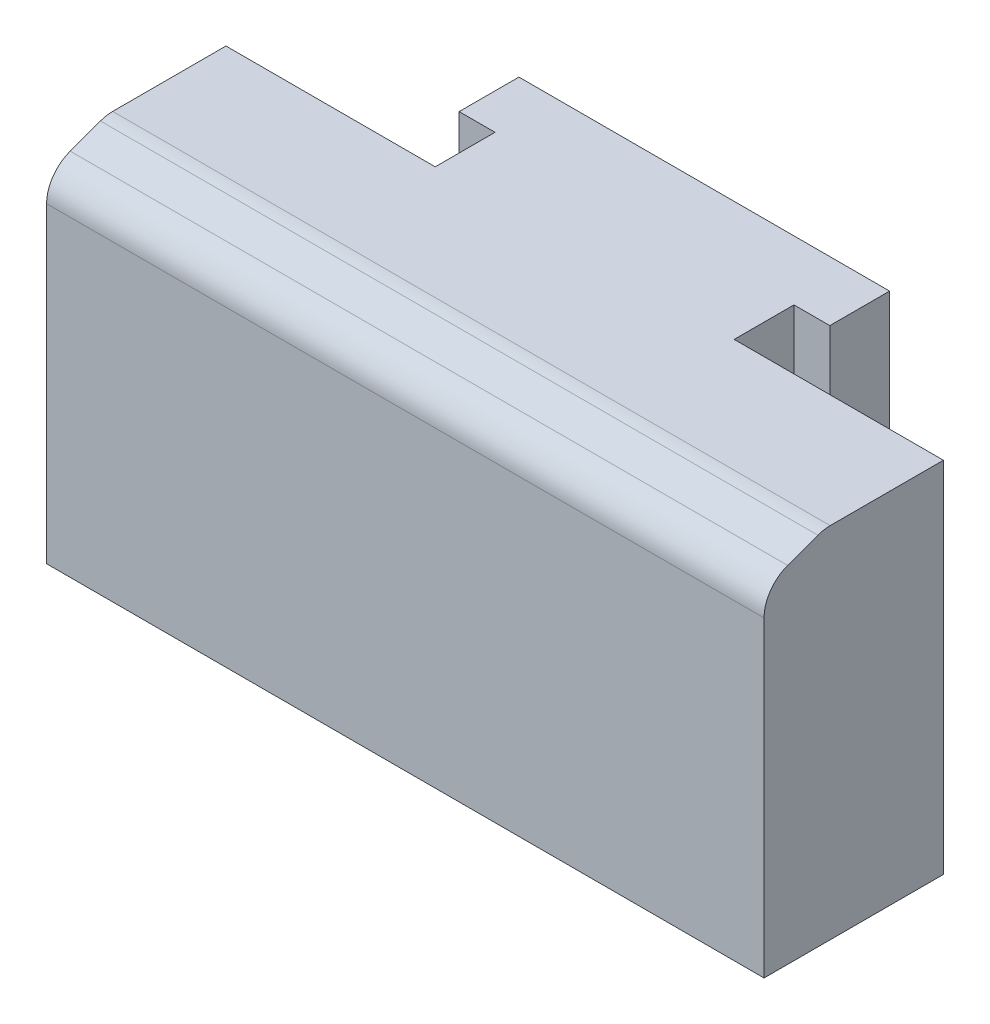
SolidWorks part; units mm, degrees
ref_plane "Front Plane" through (0, 0, 0) normal (0, 0, 1) x (1, 0, 0)
ref_plane "Top Plane" through (0, 0, 0) normal (0, 1, 0) x (1, 0, 0)
ref_plane "Right Plane" through (0, 0, 0) normal (1, 0, 0) x (0, 0, -1)
sketch "Sketch1" plane through (0, 0, 0) normal (0, 0, 1) x (1, 0, 0)
  line L1 (-32.0165, 30.1974) -> (-1.0165, 30.1974)
  line L2 (-32.0165, 30.1974) -> (-32.0165, 0.1974)
  line L3 (-32.0165, 0.1974) -> (-1.0165, 0.1974)
  line L4 (-1.0165, 30.1974) -> (-1.0165, 0.1974)
  dimension "D1" = 30
  dimension "D2" = 31
extrude "Boss-Extrude1" add sketch "Sketch1" along normal blind 25
sketch "Sketch2" plane through (0, 0.1974, 0) normal (0, -1, 0) x (1, 0, 0)
  line L0 (-32.0165, 25) -> (-1.0165, 25) construction
  line L5 (-16.5165, 0) -> (-16.5165, 13.8579) construction
  line L6 (-32.0165, 0) -> (-1.0165, 0) construction
  line L8 (-29.0165, 5) -> (-32.0165, 5)
  line L9 (-29.0165, 5) -> (-29.0165, 25)
  line L10 (-29.0165, 25) -> (-32.0165, 25)
  line L11 (-32.0165, 5) -> (-32.0165, 25)
  line L12 (-4.0165, 5) -> (-1.0165, 5)
  line L13 (-4.0165, 5) -> (-4.0165, 25)
  line L14 (-4.0165, 25) -> (-1.0165, 25)
  line L15 (-1.0165, 5) -> (-1.0165, 25)
  dimension "D1" = 25
extrude "Cut-Extrude1" cut sketch "Sketch2" against normal through all
sketch "Sketch3" plane through (0, 30.1974, 0) normal (0, 1, 0) x (1, 0, 0)
  line L1 (-4.0165, -25) -> (13.4835, -25)
  line L2 (-4.0165, -25) -> (-4.0165, -10)
  line L3 (-4.0165, -10) -> (13.4835, -10)
  line L4 (13.4835, -25) -> (13.4835, -10)
  line L5 (-29.0165, -25) -> (-46.5165, -25)
  line L6 (-29.0165, -25) -> (-29.0165, -10)
  line L7 (-29.0165, -10) -> (-46.5165, -10)
  line L8 (-46.5165, -25) -> (-46.5165, -10)
extrude "Boss-Extrude2" add sketch "Sketch3" against normal through all
chamfer "Chamfer1" distance 5 angle 20 1 edges at (-16.5165, 30.1974, 25)
fillet "Fillet1" radius 3 2 edges at (-16.5165, 28.3775, 25) (-16.5165, 30.1974, 20)
hole_wizard "M10 Tapped Hole1" positions "Sketch4" profile "Sketch5" tap size "M10" standard "ISO"
sketch "Sketch4" plane through (0, 0.1974, 0) normal (0, -1, 0) x (-1, 0, 0)
  line L0 (16.5165, -25) -> (16.5165, 0) construction
  line L1 (46.5165, -25) -> (-13.4835, -25) construction
  line L2 (32.0165, 0) -> (1.0165, 0) construction
  point P0 (16.5165, -10)
  dimension "D1" = 10
sketch "Sketch5" plane through (-16.5165, 0.1974, 10) normal (1, 0, 0) x (0, 0, -1)
  line L0 (0, 0) -> (0, 27.0537)
  line L1 (0, 27.0537) -> (4.25, 24.5)
  line L2 (4.25, 24.5) -> (4.25, 0)
  line L5 (4.25, 0) -> (0, 0)
  line L10 (0, 27.0537) -> (-4.25, 24.5) construction
  line L11 (0, -6.35) -> (0, 107.95) construction
  dimension "螺纹孔钻头直径" = 8.5
  dimension "螺纹孔钻头深度" = 24.5
  dimension "导头角度" = 118
cosmetic thread "Hole Thread 1" parameters "D1"=20, "D2"=10
